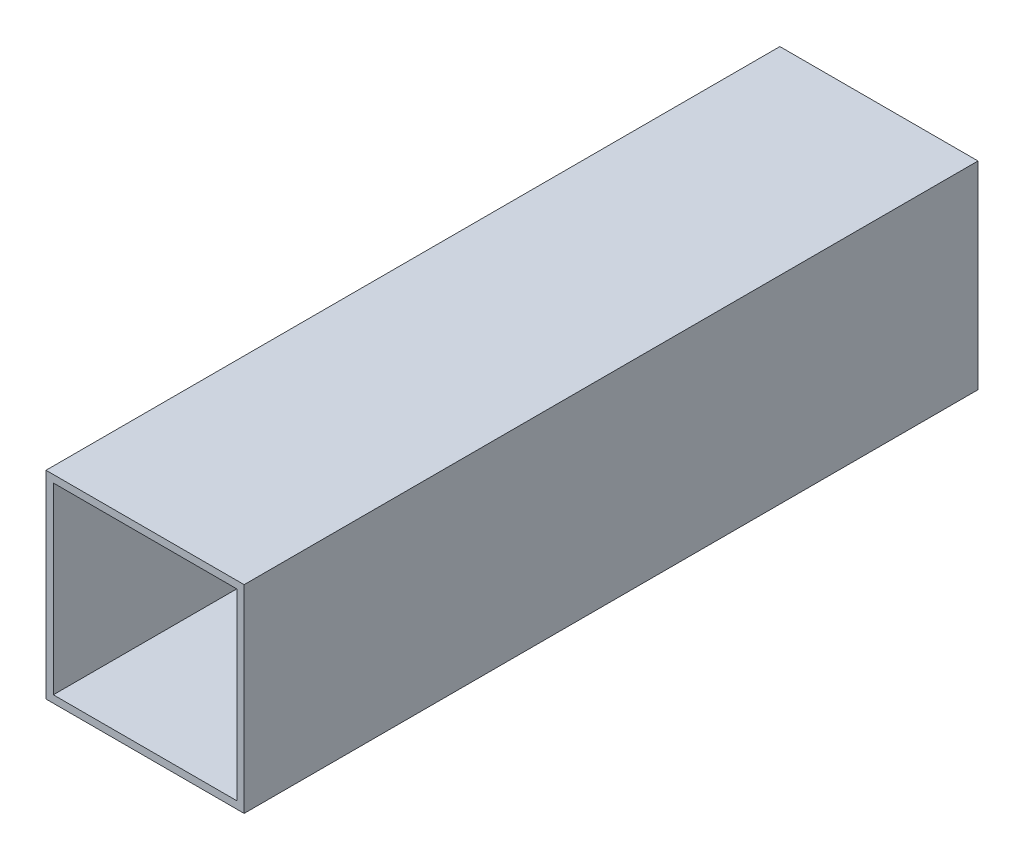
SolidWorks part; units mm, degrees
ref_plane "Front Plane" through (0, 0, 0) normal (0, 0, 1) x (1, 0, 0)
ref_plane "Top Plane" through (0, 0, 0) normal (0, 1, 0) x (1, 0, 0)
ref_plane "Right Plane" through (0, 0, 0) normal (1, 0, 0) x (0, 0, -1)
sketch "Sketch1" plane through (0, 0, 0) normal (0, 0, 1) x (1, 0, 0)
  line L1 (125, 125) -> (-125, 125)
  line L2 (125, 125) -> (125, -125)
  line L3 (125, -125) -> (-125, -125)
  line L4 (-125, 125) -> (-125, -125)
  line L5 (125, 125) -> (-125, -125) construction
  line L6 (125, -125) -> (-125, 125) construction
  point P0 (0, 0)
  dimension "D1" = 250
extrude "Extrude-Thin1" add sketch "Sketch1" along normal blind 1000 thin
